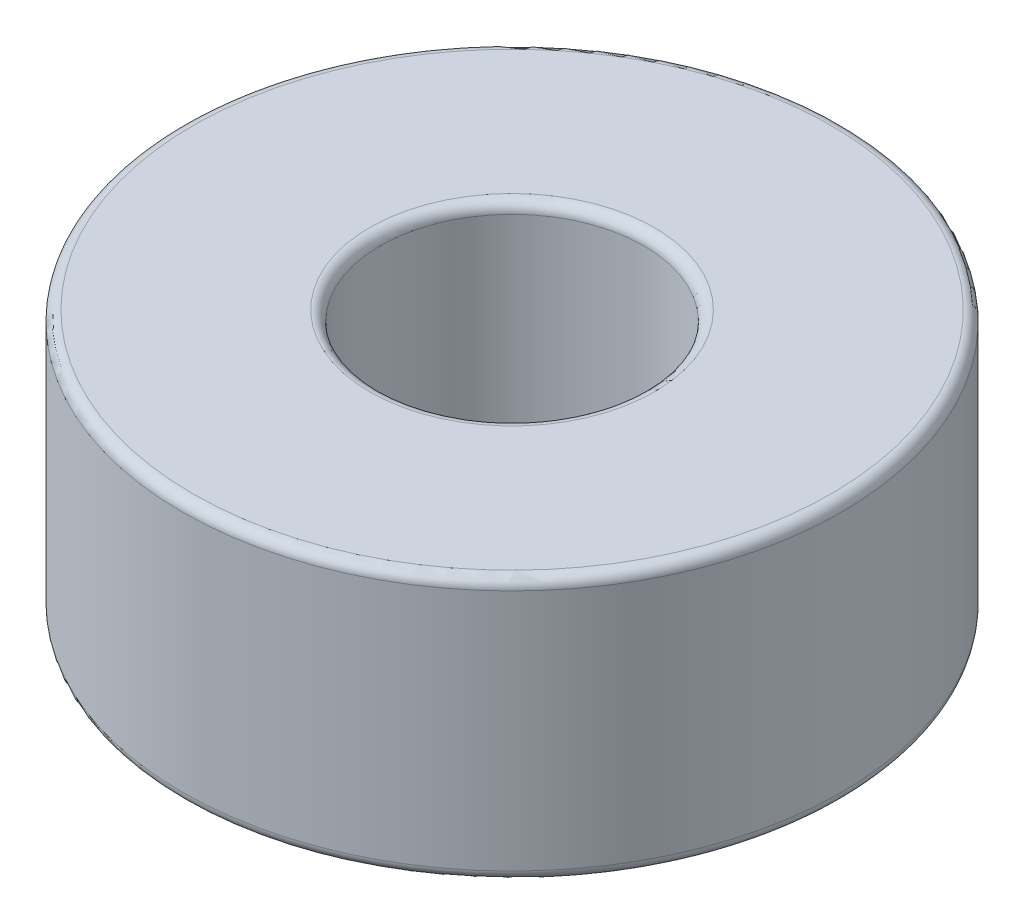
from build123d import *

# Parameters (mm, degrees)
SKETCH_1_R       = 2.5
SKETCH_1_R_2     = 1
EXTRUDE_1_DEPTH  = 2
FILLET_R0_08_1_R = 0.08


with BuildPart() as part:
    # 草图1 → 凸台-拉伸1 (new body)
    with BuildSketch(Plane(origin=(0, 0, 0), x_dir=(1, 0, 0), z_dir=(0, 1, 0))):
        with Locations(Location((0, 0, 0), (0, 0, 270))):
            Circle(SKETCH_1_R)
        with Locations(Location((0, 0, 0), (0, 0, 270))):
            Circle(SKETCH_1_R_2, mode=Mode.SUBTRACT)
    extrude(amount=EXTRUDE_1_DEPTH)

    # R0.08 圆角1
    fillet_r0_08_1_edges = [part.edges().sort_by_distance(p)[0] for p in [
        (0, 0, -2.5),
        (0, 2, -2.5),
        (0, 0, -1),
        (0, 2, -1),
    ]]
    fillet(fillet_r0_08_1_edges, radius=FILLET_R0_08_1_R)


solid = part.part
